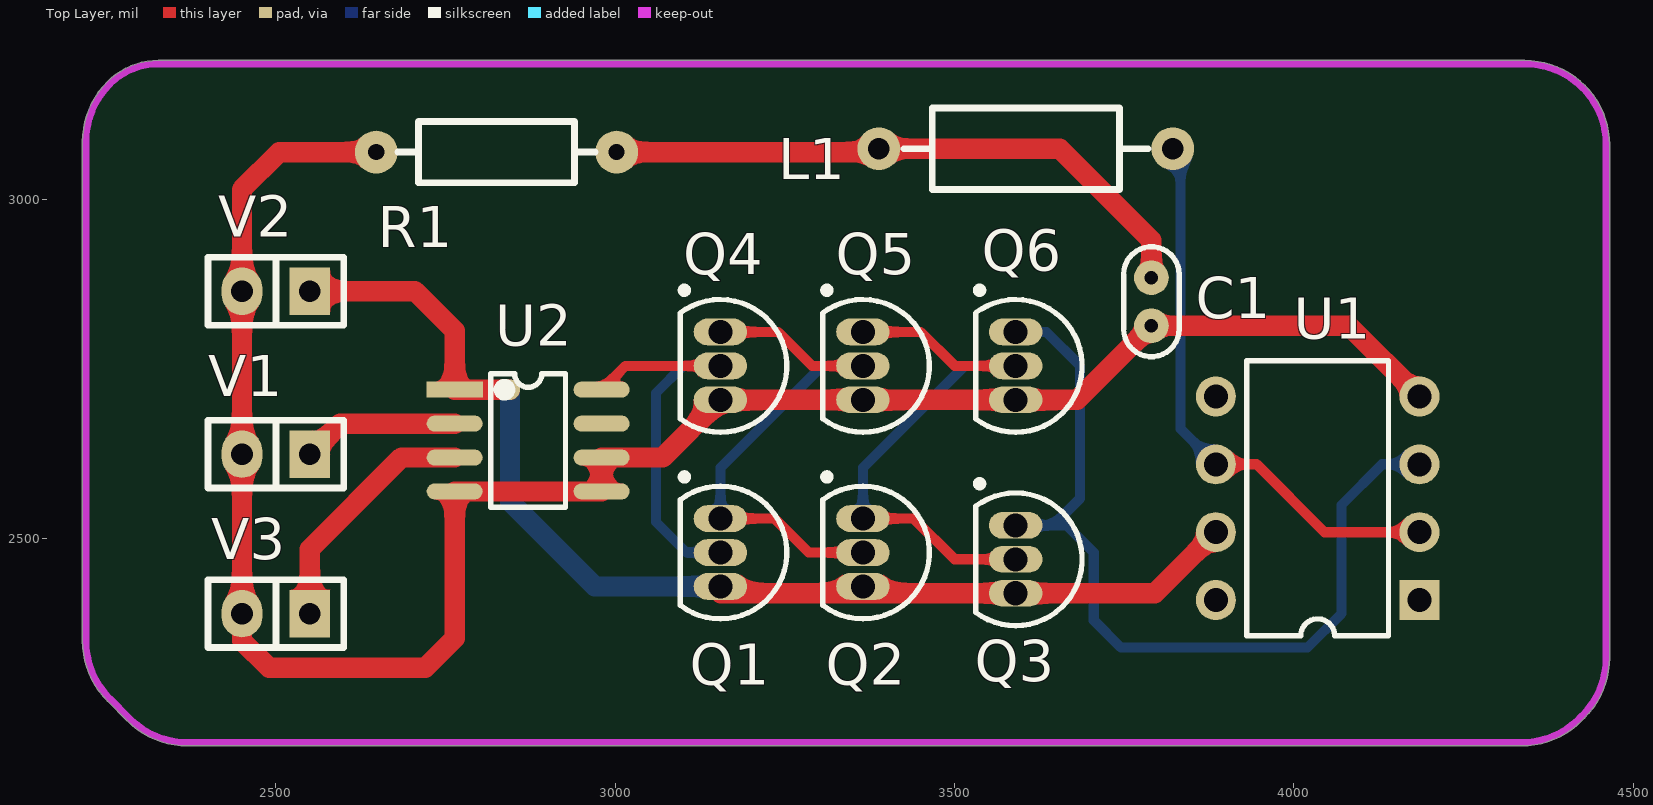
[diagram p0: Top Layer view]
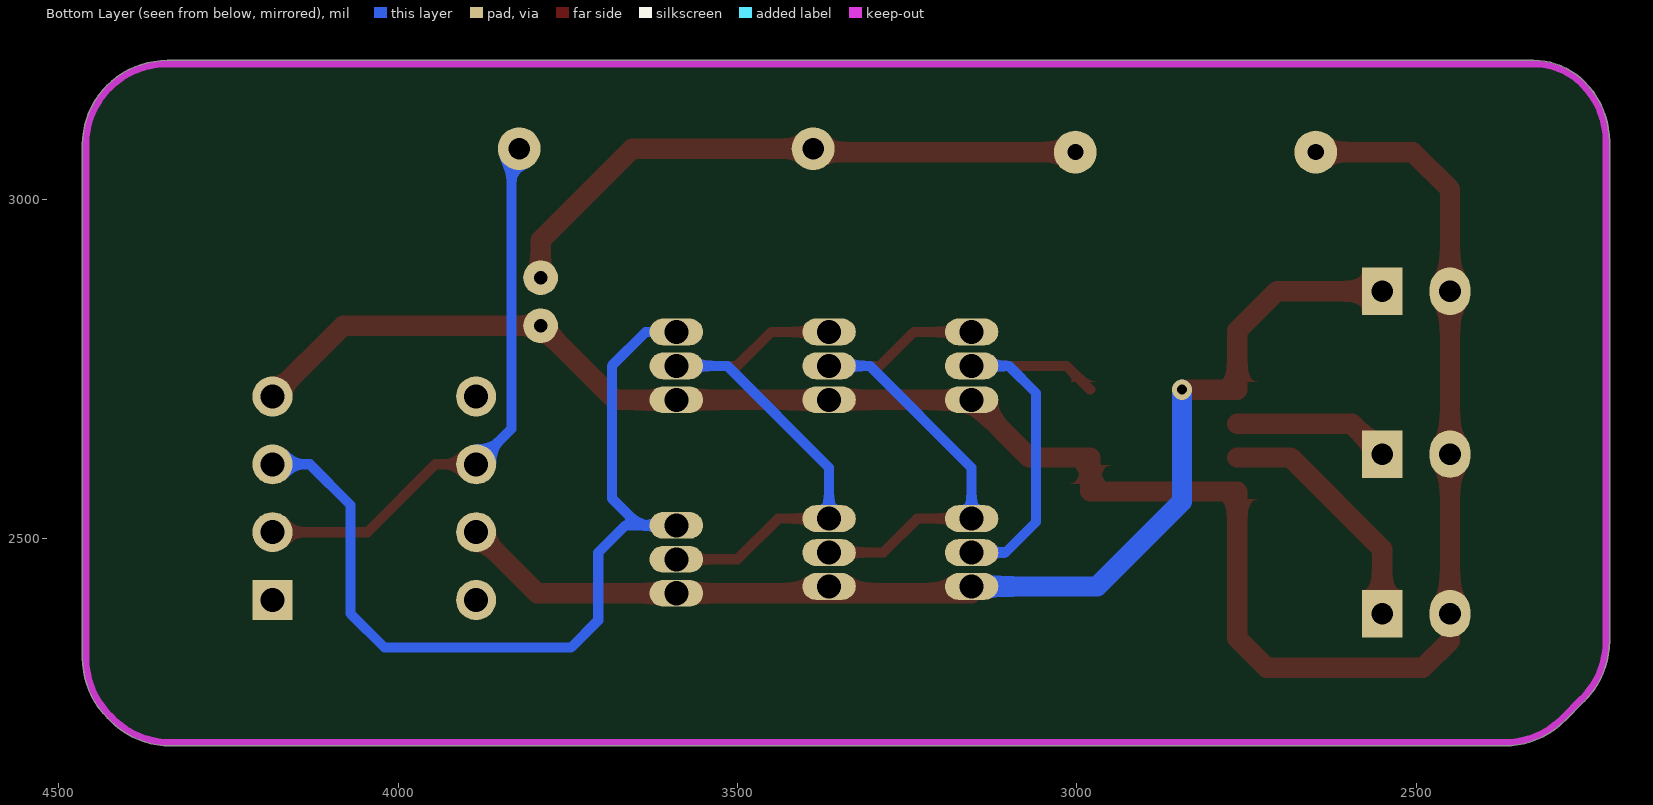
[diagram p1: Bottom Layer view, seen from below]
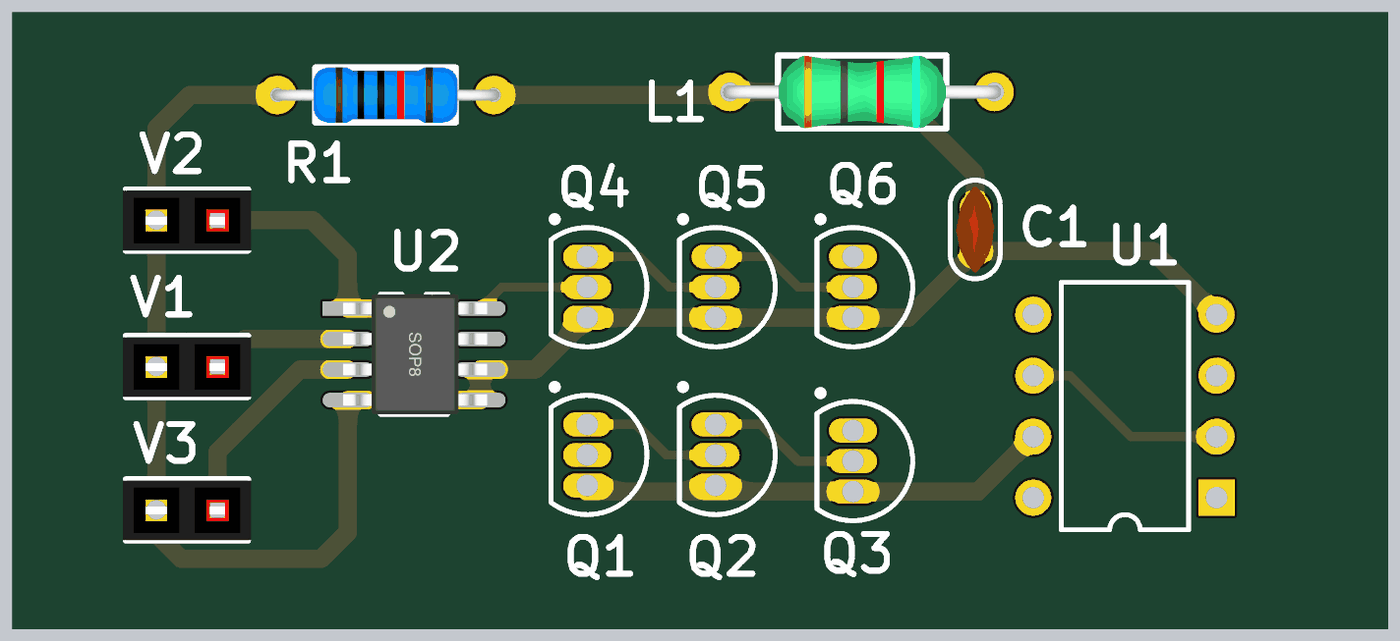
[diagram p2: 3D render of the assembled board from above, using the file's embedded part models]
# Altium PCB MISC80654.PcbDoc
Units mil, origin at the board's own origin, x right, y up, seen from the top; angles counter-clockwise.
Board outline 2250.03 x 1010.03 mil, 2 copper layers (Top Layer, Bottom Layer); 14 components, 10 nets, 46 pads, 1 vias.

## Layer stack, top to bottom (the 12.6 mil dielectric is the usual default, probably not edited)
Top Solder: solder mask 0.4, Solder Resist, Dk 3.5
Top Layer: signal copper 1.4
Dielectric 1: dielectric 12.6, FR-4, Dk 4.8
Bottom Layer: signal copper 1.4
Bottom Solder: solder mask 0.4, Solder Resist, Dk 3.5

## Board outline
2281.08,2231.83 ccw(c2284.64,2235.36) 2281.1,2231.81 2251.81,2261.1 cw(c2340.71,2350) 2214.99,2350 2214.99,3085 cw(c2340.71,3085) 2251.81,3173.9 cw(c2326.92,3098.79) 2326.92,3205.01 4340,3205.01 cw(c4340,3079.29) 4428.9,3168.19 cw(c4341.72,3081.01) 4465.02,3081.01 4465.02,2325 cw(c4339.29,2325) 4428.19,2236.1 cw(c4424.64,2239.64) 4428.17,2236.08 4428.19,2236.1 4423.9,2231.81 ccw(c4420.36,2235.36) 4423.92,2231.83 4423.9,2231.81 cw(c4335,2320.71) 4335,2194.99 2370,2194.99 cw(c2370,2320.71)

## Design rules (kind name [scope] priority, off if disabled: settings)
Clearance [All] p1: gap=10
MinimumSolderMaskSliver [All] p1: minsoldermaskwidth=0
PolygonConnect [All] p1: connectstyle=Relief reliefconductorwidth=10 reliefentries=4 polygonreliefangle="90 Angle" airgapwidth=10
RoutingVias [All] p1: holewidth=28 width=50 viastyle="Through Hole" minholewidth=28 minwidth=50 maxholewidth=28 maxwidth=50
SilkToSilkClearance [All] p1: silktosilkclearance=0
SilkToSolderMaskClearance [IsPad] p1: minsilkscreentomaskgap=0 clearancetoexposedcopper=TRUE
SolderMaskExpansion [All] p1: expansion=4
Width [All] p1: maxlimit=30 minlimit=10 preferedwidth=10
27 further rules are at their usual default settings.

## Components (designator, comment, footprint, x,y, rotation, side; value= is the part's Value field where it differs from the comment)
C1 "0.47U" "CC 1.8*3.6" 3790,2849.57 r270 top
L1 "2.2MH" AL0307 3605,3075 r180 top
Q1 "2N3904" TO-92A 3155,2480 r180 top
Q2 "2N3904" TO-92A 3365,2480 r180 top
Q3 "2N3904" TO-92A 3590,2470 r180 top
Q4 "2N3906" TO-92A 3155,2755 r180 top
Q5 "2N3906" TO-92A 3365,2755 r180 top
Q6 "2N3906" TO-92A 3590,2755 r180 top
R1 "47" "RS 1/4W" 2825,3070 r0 top
U1 "OP177AZ" Q-8 4035,2560 r90 top
U2 "LT1711" SOP8 2763.46,2720 r0 top
V1 "Current source" Fe-HDR1X2/2.54-S 2550,2625 r180 top
V2 "Current source" Fe-HDR1X2/2.54-S 2550,2865 r180 top
V3 "Female HDR1X2" Fe-HDR1X2/2.54-S 2550,2390 r180 top

## Footprints (in the part's own frame and the unit in brackets; to place one, negate y for a bottom-side part, rotate by r counter-clockwise, add the part's x,y. Pads: shape width x height; smd on the part's side, far side on the other; paste and mask are expansions set on the pad)
AL0307 [mm] "11*3*7mm（脚距，直径，长度）"
  round 1.6 hole 0.8: 1(-5.5,0) 2(5.5,0)
  silkscreen extent -4.57,-1.52 4.57,1.52, body extent -5.78,-1.51 5.78,1.51, height 3.06
"CC 1.8*3.6" [mm] "脚距1.8mm直径3.6mm"
  round 1.3 hole 0.5: 1(-0.9,0) 2(0.9,0)
  silkscreen extent -2.05,-1.04 2.05,1.04, body extent -1.8,-0.8 1.8,0.8, height 3.6
Fe-HDR1X2/2.54-S [mil] "Connector; Header; 2x2 Position"
  rect 60x70 hole 32: 1(0,0)
  oval 60x70 hole 32: 2(100,0)
  silkscreen extent -50,-50 150,50, body extent -55,-48 155,50, height 335
Q-8 [mm] "DIP; 8 Leads; Row Spacing 7.62 mm; Pitch 2.54 mm"
  rect 1.5x1.5 hole 0.9: 1(-3.81,-3.81)
  round 1.5 hole 0.9: 2(-1.27,-3.81) 3(1.27,-3.81) 4(3.81,-3.81) 5(3.81,3.81) 6(1.27,3.81) 7(-1.27,3.81) 8(-3.81,3.81)
  silkscreen extent -5.15,-2.65 5.15,2.65
"RS 1/4W" [mm] "直插色环电阻，脚距9mm，直径2.3mm"
  round 1.6 hole 0.6: 1(-4.5,0) 2(4.5,0)
  silkscreen extent -3.68,-1.14 3.68,1.14, body extent -4.72,-1.16 4.73,1.16, height 2.32
SOP8 [mm]
  rect 2.1x0.6 smd: 1(0,0)
  oval 2.1x0.6 smd: 2(0,-1.27) 3(0,-2.54) 4(0,-3.81) 5(5.5,-3.81) 6(5.5,-2.54) 7(5.5,-1.27) 8(5.5,0)
  silkscreen extent 1.35,-4.41 4.15,0.6, body extent -0.21,-4.4 5.8,0.6, height 1.9
TO-92A [mm] "TO, Flat Index; 3 In-Line, Axial Leads; Body Dia. 4.5mm; Leads 0.51 x 0.48 mm (max)"
  oval 2x1 hole 0.9: 1(0,-1.27) 2(0,0) 3(0,1.27)
  silkscreen extent -2.48,-2.95 1.5,2.48, body extent -2.48,-2.5 1.5,2.5, height 6.86

## Part data
C1: library part CC, "Ceramic disc capacitor"
L1: library part L-AL, "Color-band inductor"
Q1 Q2 Q3: "NPN General Purpose Amplifier"
Q4 Q5 Q6: "PNP General Purpose Amplifier"
R1: library part R-S, "Color-band resistor"
U1: "Ultraprecision Operational Amplifier"
U2: library part LT1711CMS8#PBF
V1 V2: library part 电流源

## Via types
v1: diameter 30, hole 15, Top Layer to Bottom Layer, 1 vias

## Nets (pads, with @x,y where several pads share a name; then routed paths per layer and width w, separated by ;. In a path a pad name is that pad's centre, name@x,y a point inside that pad or via, vN(x,y) a via of type N, cw(c..) or ccw(c..) an arc to the next point about the centre after c; other vN are vias at no path point)
GND: C1.2 Q4.3 Q5.3 Q6.3 R1.1 U1.4 U2.4 U2.5 U2.6 V1.2 V2.2 V3.2 | length 3045.3
  Top Layer w30: R1.1 2505,3070 2450,3015 V2.2 V1.2 V3.2 2450,2350 2490,2310 2720,2310 2763.46,2353.46 U2.4 U2.5 U2.6 3070,2620 Q4.3 Q5.3 Q6.3 3680.87,2705 C1.2 4080.87,2814.13 U1.4
NetC1_1: C1.1 L1.2 R1.2 | length 900.8
  Top Layer w30: R1.2 3383.46,3070 L1.2 3655,3075 3790,2940 C1.1
NetL1_1: L1.1 U1.2 U1.6 | length 832.7
  Top Layer w15: U1.6 3945,2610 4045,2510 U1.2
  Bottom Layer w15: L1.1 3833.09,3063.44 3833.09,2661.91 U1.6
NetQ1_1: Q1.1 Q2.2 Q4.1 Q5.2 | length 808.6
  Top Layer w15: Q1.1 3235,2530 3285,2480 Q2.2 ; Q4.1 3240,2805 3290,2755 Q5.2
  Bottom Layer w15: Q1.1 3155,2605 3305,2755 Q5.2
NetQ1_2: Q1.2 Q4.2 U2.8 | length 604.7
  Top Layer w15: U2.8 3015,2755 Q4.2
  Bottom Layer w15: Q1.2 3105,2480 3060,2525 3060,2715 3100,2755 Q4.2
NetQ2_1: Q2.1 Q3.2 Q5.1 Q6.2 | length 857.7
  Top Layer w15: Q2.1 3440,2530 3500,2470 Q3.2 ; Q5.1 3450,2805 3500,2755 Q6.2
  Bottom Layer w15: Q2.1 3365,2605 3515,2755 Q6.2
NetQ3_1: Q3.1 Q6.1 U1.3 | length 1301
  Bottom Layer w15: Q3.1 3645,2520 ; Q6.1 3635,2805 3685,2755 3685,2560 3645,2520 ; U1.3 4130,2610 4070,2550 4070,2390 4020,2340 3745,2340 3705,2380 3705,2480 3665,2520 3645,2520
NetU2_2: U2.2 V1.1 | length 232.1
  Top Layer w30: V1.1 2595,2670 U2.2
NetU2_3: U2.3 V3.1 | length 364.4
  Top Layer w30: V3.1 2550,2485 2685,2620 U2.3
VCC: Q1.3 Q2.3 Q3.3 U1.7 U2.1 V2.1 | length 1719.8
  Top Layer w30: V2.1 2705,2865 2763.46,2806.54 U2.1 v1(2845,2720) ; Q1.3 3155,2420 Q2.3@3365,2420 ; Q2.3 Q2.3@3365,2420 ; U1.7 3795,2420 Q3.3 Q2.3@3365,2420
  Bottom Layer w30: v1(2845,2720) 2845,2555 2970,2430 Q1.3
pads on no net: U1.1 U1.5 U1.8 U2.7

## Keep-outs
Keep-Out Layer:
  lines w10: 2600,3200 4340,3200 cw(c4340,3079.29) 4425.36,3164.64 cw(c4341.72,3081.01) 4460,3081.01 4460,2325 cw(c4339.29,2325) 4424.64,2239.64 4420.36,2235.36 cw(c4335,2320.71) 4335,2200 2370,2200 cw(c2370,2320.71) 2284.64,2235.36 2255.36,2264.64 cw(c2340.71,2350) 2220,2350 2220,3085 cw(c2340.71,3085) 2255.36,3170.36 cw(c2326.92,3098.79) 2326.92,3200 2680,3200